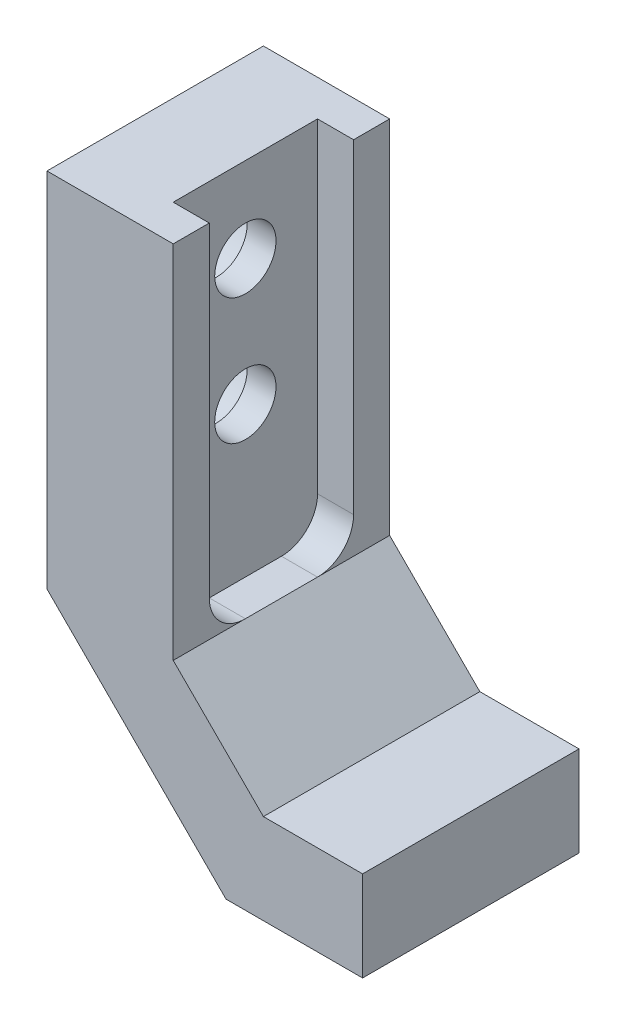
SolidWorks part; units mm, degrees
ref_plane "前视基准面" through (0, 0, 0) normal (0, 0, 1) x (1, 0, 0)
ref_plane "上视基准面" through (0, 0, 0) normal (0, 1, 0) x (1, 0, 0)
ref_plane "右视基准面" through (0, 0, 0) normal (1, 0, 0) x (0, 0, -1)
sketch "草图1" plane through (0, 0, 0) normal (0, 0, 1) x (1, 0, 0)
  line L0 (0, 0) -> (0, -20.0711)
  line L1 (0, -20.0711) -> (9.9289, -30)
  line L3 (12, -25) -> (7, -20)
  line L4 (7, -20) -> (7, 0)
  line L5 (7, 0) -> (0, 0)
  line L6 (12, -25) -> (17.5, -25)
  line L7 (17.5, -25) -> (17.5, -30)
  line L8 (17.5, -30) -> (9.9289, -30)
  dimension "D1" = 5
  dimension "D2" = 20
  dimension "D3" = 7
  dimension "D4" = 10.5
  dimension "D5" = 135
  dimension "D6" = 5
  dimension "D7" = 10
extrude "凸台-拉伸1" add sketch "草图1" along normal mid plane 12
sketch "草图2" plane through (0, 0, 0) normal (0, 1, 0) x (1, 0, 0)
  line L0 (7, -6) -> (7, 6) construction
  line L1 (7, 4) -> (5, 4)
  line L2 (7, 4) -> (7, -4)
  line L3 (7, -4) -> (5, -4)
  line L4 (5, 4) -> (5, -4)
  point P6 (5, 0)
  dimension "D1" = 8
  dimension "D2" = 2
extrude "切除-拉伸1" cut sketch "草图2" against normal blind 20
fillet "圆角1" radius 2
sketch "草图5" plane through (0, 0, 0) normal (-1, 0, 0) x (0, 0, 1)
  point P0 (0, -4.7)
  point P3 (0, -11.7)
hole_wizard "M3 六角圆柱头螺钉的柱形沉头孔1" positions "草图5" profile "草图4" counterbore size "M3" standard "GB" end condition through all
sketch "草图4" plane through (0, -4.7, 0) normal (0, 1, 0) x (0, 0, 1)
  line L0 (0, 0) -> (0, 17.5)
  line L1 (0, 17.5) -> (1.7, 17.5)
  line L3 (1.7, 17.5) -> (1.7, 3.4)
  line L4 (1.7, 3.4) -> (3, 3.4)
  line L5 (3, 3.4) -> (3, 0)
  line L7 (3, 0) -> (0, 0)
  line L11 (0, -6.35) -> (0, 107.95) construction
  dimension "通孔孔直径" = 3.4
  dimension "通孔孔深度" = 17.5
  dimension "柱形沉头孔直径" = 6
  dimension "柱形沉头孔深度" = 3.4
